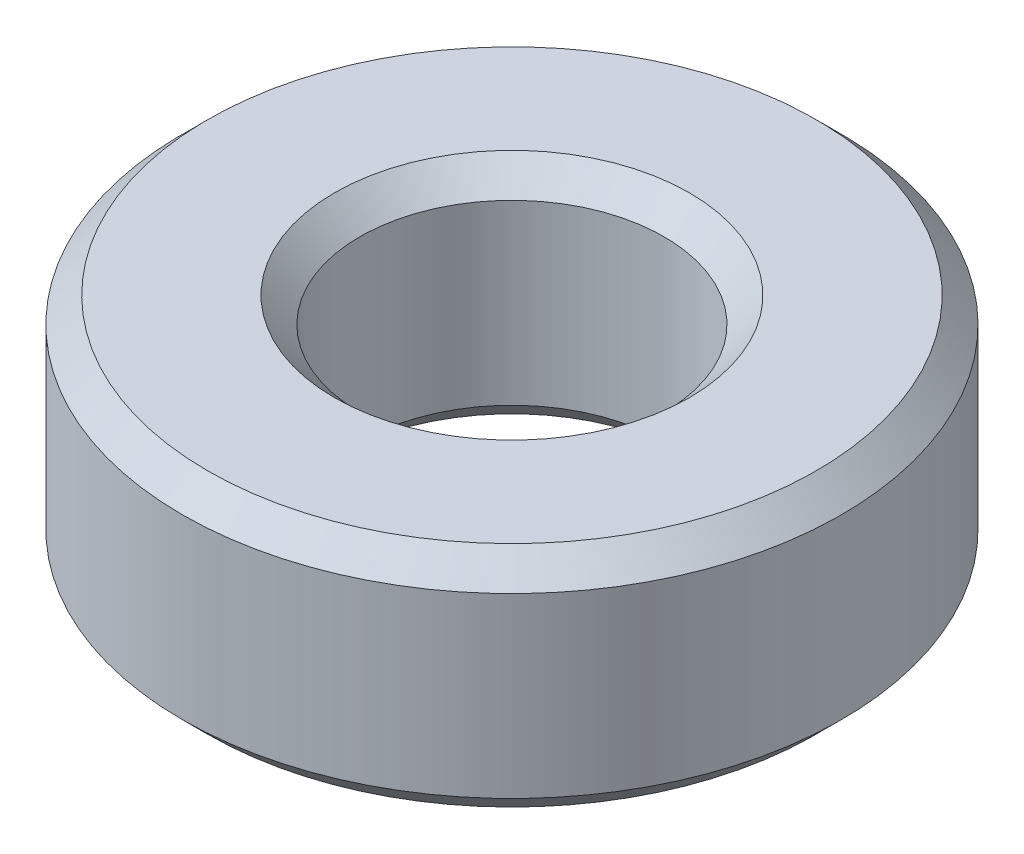
from build123d import *

# Parameters (mm, degrees)
SKETCH1_R           = 6.5
SKETCH1_R_2         = 3
BOSS_EXTRUDE1_DEPTH = 4.5
CHAMFER1_SIZE       = 0.5


with BuildPart() as part:
    # Sketch1 → Boss-Extrude1 (new body)
    with BuildSketch(Plane(origin=(0, 0, 0), x_dir=(1, 0, 0), z_dir=(0, 1, 0))):
        with Locations(Location((0, 0, 0), (0, 0, 270))):
            Circle(SKETCH1_R)
        with Locations(Location((0, 0, 0), (0, 0, 270))):
            Circle(SKETCH1_R_2, mode=Mode.SUBTRACT)
    extrude(amount=BOSS_EXTRUDE1_DEPTH)

    # Chamfer1
    chamfer1_edges = [part.edges().sort_by_distance(p)[0] for p in [
        (0, 0, -6.5),
        (0, 4.5, -6.5),
        (0, 0, -3),
        (0, 4.5, -3),
    ]]
    chamfer(chamfer1_edges, length=CHAMFER1_SIZE)


solid = part.part
